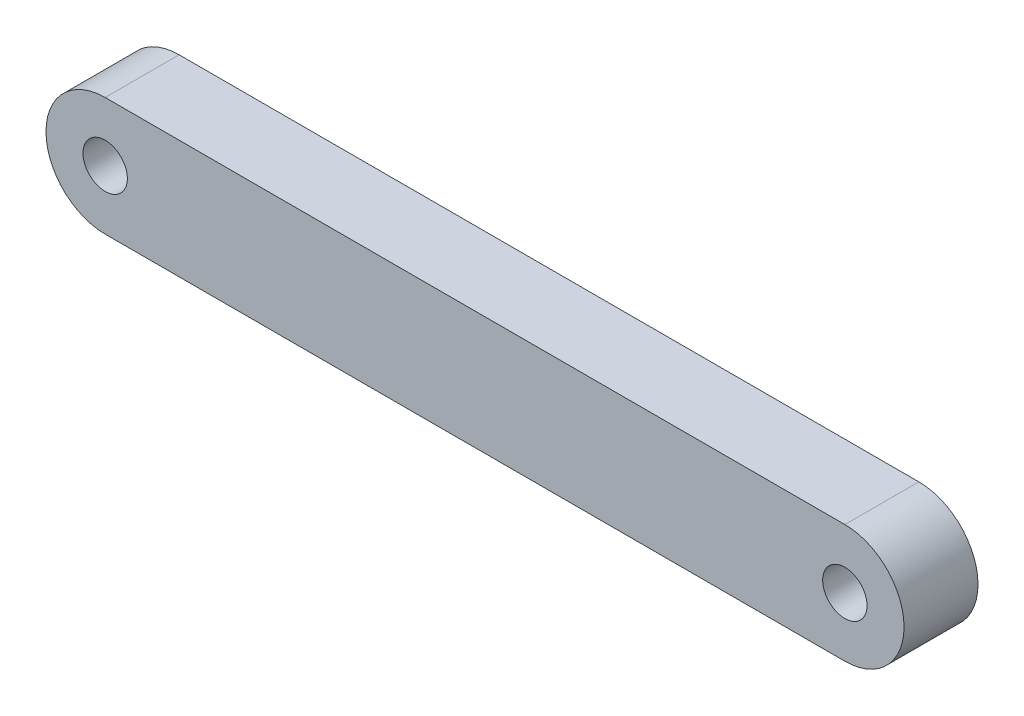
SolidWorks part; units mm, degrees
material "1.0503 (C45)"
ref_plane "Front Plane" through (0, 0, 0) normal (0, 0, 1) x (1, 0, 0)
ref_plane "Top Plane" through (0, 0, 0) normal (0, 1, 0) x (1, 0, 0)
ref_plane "Right Plane" through (0, 0, 0) normal (1, 0, 0) x (0, 0, -1)
sketch "Sketch1" plane through (0, 0, 0) normal (0, 0, 1) x (1, 0, 0)
  line L0 (-25, 0) -> (25, 0) construction
  line L1 (-25, 4) -> (25, 4)
  line L2 (-25, -4) -> (25, -4)
  arc A0 (-25, 4) -> (-25, -4) centre (-25, 0) ccw
  arc A1 (25, -4) -> (25, 4) centre (25, 0) ccw
  point P2 (0, 0)
  dimension "D2" = 4
  dimension "D1" = 50
extrude "Boss-Extrude1" add sketch "Sketch1" along normal blind 5
sketch "Sketch3" plane through (0, 0, 5) normal (0, 0, 1) x (1, 0, 0)
  circle A0 centre (-25, 0) radius 1.5
  circle A1 centre (25, 0) radius 1.5
  arc A2 (-25, 4) -> (-25, -4) centre (-25, 0) ccw construction
  arc A3 (25, -4) -> (25, 4) centre (25, 0) ccw construction
  dimension "D1" = 3
extrude "Cut-Extrude1" cut sketch "Sketch3" against normal through all
